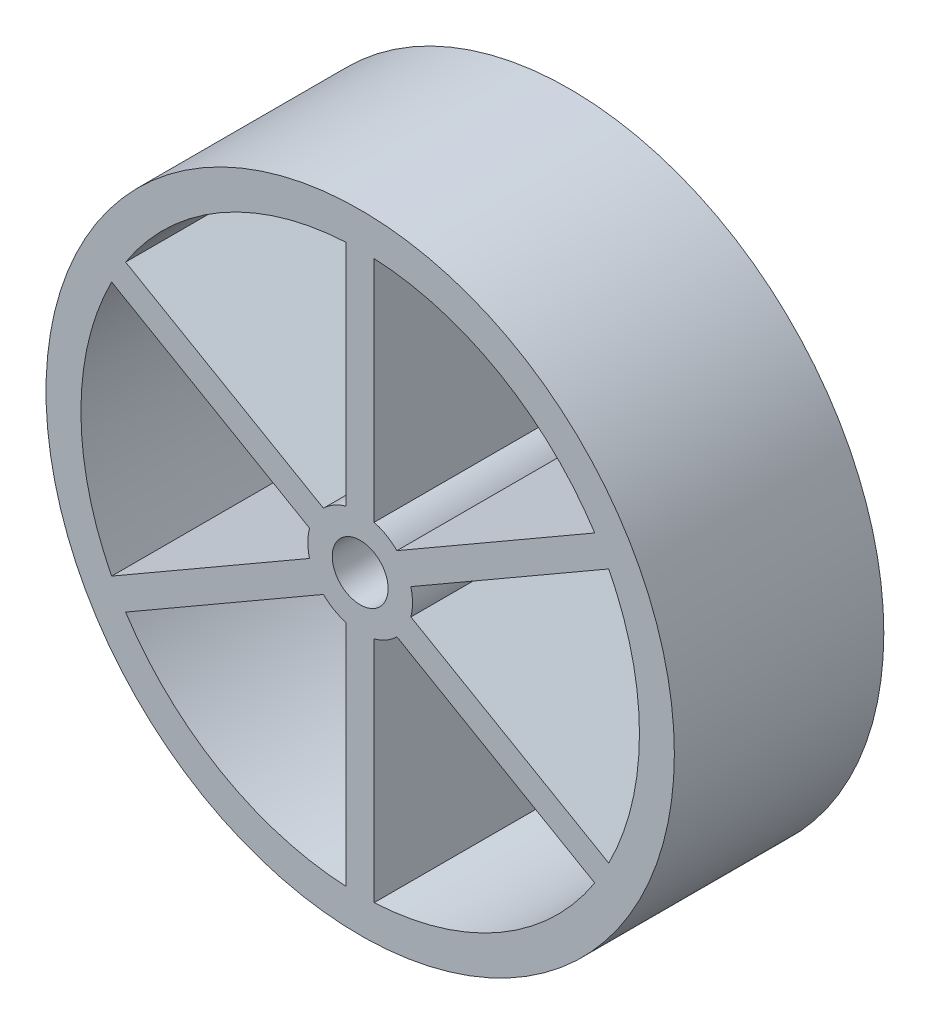
from build123d import *

# Parameters (mm, degrees)
SKETCH1_R               = 7.5
BOSS_EXTRUDE1_DEPTH     = 30
SKETCH2_R               = 45
SKETCH2_R_2             = 40
EXTRUDE_THIN1_DEPTH     = 30
SKETCH5_W               = 4
SKETCH5_H               = 36.329230713
EXTRUDE_THIN3_DEPTH     = 30
CIRPATTERN4_COUNT       = 6
CUT_EXTRUDE1_DEPTH      = 124.778996688
CUT_EXTRUDE1_DEPTH_BACK = 124.778996688
SKETCH6_R               = 4


with BuildPart() as part:
    # Sketch1 → Boss-Extrude1 (new body)
    with BuildSketch(Plane.XY):
        with Locations((10, -61.753173354)):
            Circle(SKETCH1_R)
    extrude(amount=BOSS_EXTRUDE1_DEPTH)



with BuildPart() as body_2:
    # Sketch2 → Extrude-Thin1 (new body)
    with BuildSketch(Plane.XY.offset(30)):
        with Locations((10, -61.753173354)):
            Circle(SKETCH2_R)
        with Locations((10, -61.753173354)):
            Circle(SKETCH2_R_2, mode=Mode.SUBTRACT)
    extrude(amount=-EXTRUDE_THIN1_DEPTH)


with BuildPart() as part_1:
    add(part.part)

    add(body_2.part)  # Extrude-Thin3 merges body 2
    # Sketch5 → Extrude-Thin3 (add)
    with BuildSketch(Plane.XY.offset(30)):
        with Locations((10, -39.294001794)):
            Rectangle(SKETCH5_W, SKETCH5_H)
    extrude_thin3 = extrude(amount=-EXTRUDE_THIN3_DEPTH)

    # CirPattern4: Extrude-Thin3 ×6 about axis
    cirpattern4_axis = Axis((10, -61.753173354, 0), (0, 0, 1))
    for i in range(1, CIRPATTERN4_COUNT):
        add(extrude_thin3.rotate(cirpattern4_axis, i * 360 / CIRPATTERN4_COUNT))

    # Sketch6 → Cut-Extrude1 (cut, two sides: drawn at the far end of the back side and taken through both)
    with BuildSketch(Plane.XY.offset(30).offset(-CUT_EXTRUDE1_DEPTH_BACK)):
        with Locations((10, -61.753173354)):
            Circle(SKETCH6_R)
    extrude(amount=CUT_EXTRUDE1_DEPTH + CUT_EXTRUDE1_DEPTH_BACK, mode=Mode.SUBTRACT)


solid = part_1.part
